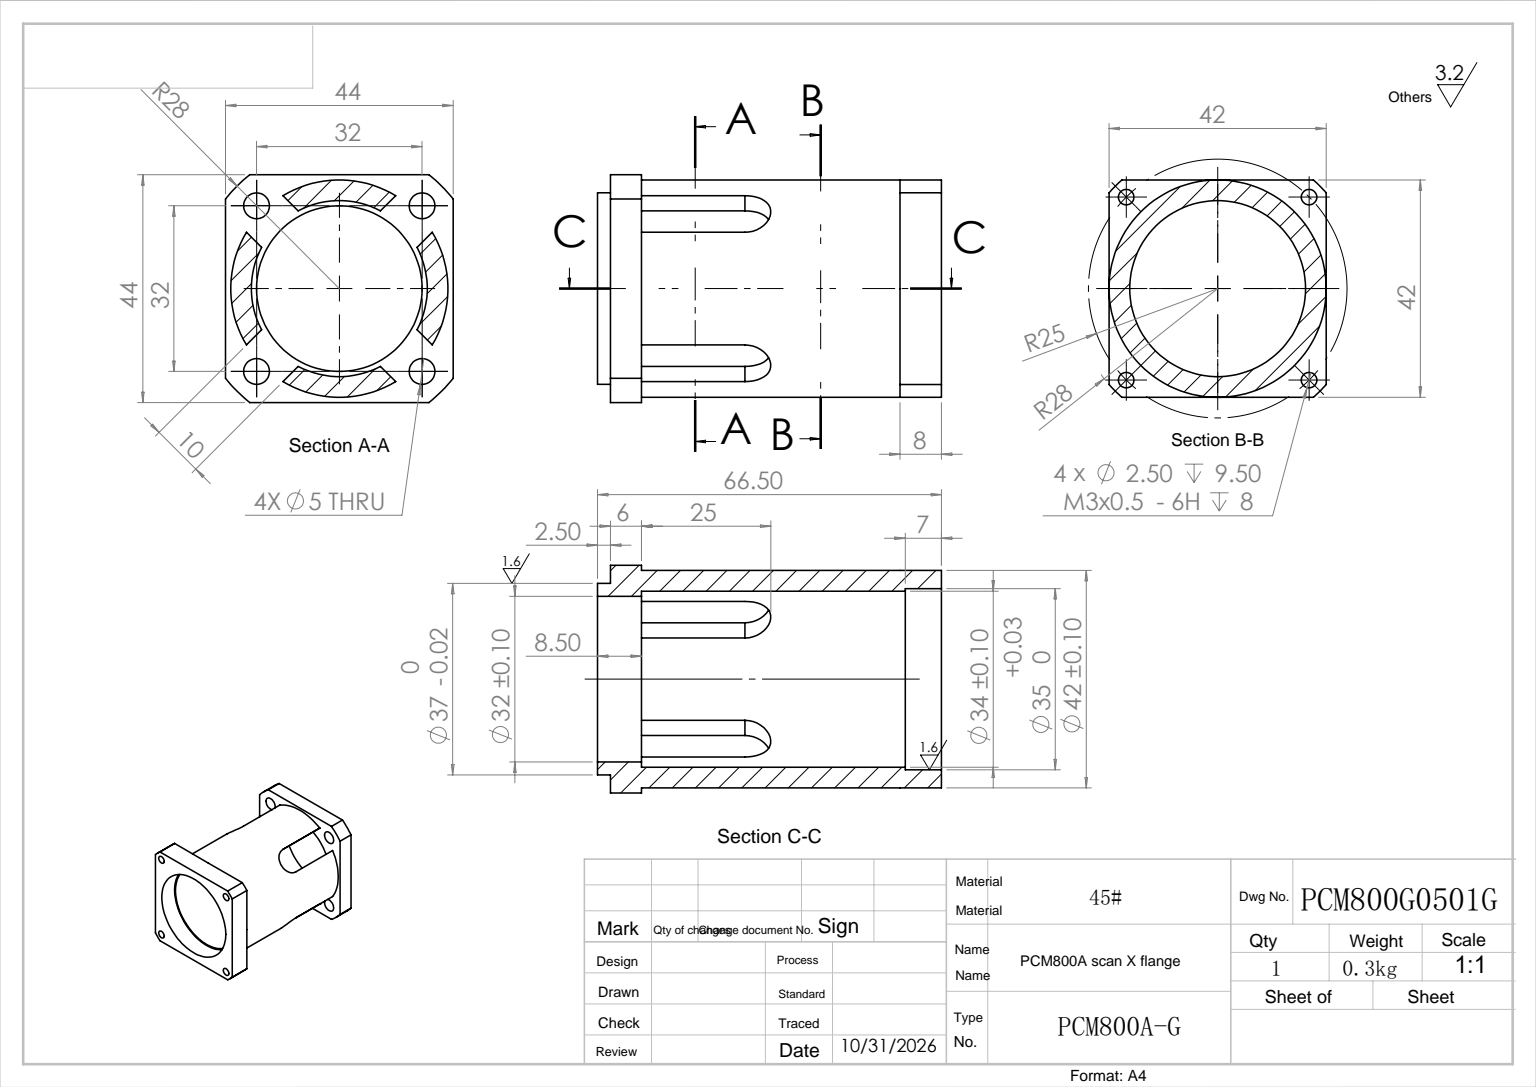
SolidWorks part; units mm, degrees
ref_plane "前视" through (0, 0, 0) normal (0, 0, 1) x (1, 0, 0)
ref_plane "上视" through (0, 0, 0) normal (0, 1, 0) x (1, 0, 0)
ref_plane "右视" through (0, 0, 0) normal (1, 0, 0) x (0, 0, -1)
sketch "草图1" plane through (0, 0, 0) normal (0, 0, 1) x (1, 0, 0)
  circle A0 centre (0, 0) radius 21
  circle A1 centre (0, 0) radius 17
  dimension "D1" = 42
  dimension "D2" = 34
extrude "拉伸1" add sketch "草图1" along normal blind 50
sketch "草图3" plane through (0, 0, 0) normal (0, 0, -1) x (-1, 0, 0)
  line L0 (0, 27.9971) -> (0, -28.1043) construction
  line L1 (-24.189, 0) -> (27.5144, 0) construction
  line L3 (-22, 22) -> (22, 22)
  line L4 (-22, 22) -> (-22, -22)
  line L5 (-22, -22) -> (22, -22)
  line L6 (22, 22) -> (22, -22)
  dimension "D1" = 22
  dimension "D2" = 22
  dimension "D3" = 44
  dimension "D4" = 44
extrude "拉伸2" add sketch "草图3" along normal blind 6
sketch "草图4" plane through (0, 0, -6) normal (0, 0, -1) x (-1, 0, 0)
  line L0 (-22, 0) -> (22, 0) construction
  line L1 (-22, 22) -> (-22, -22) construction
  line L2 (22, -22) -> (22, 22) construction
  line L3 (0, 22) -> (0, -22) construction
  line L4 (22, 22) -> (-22, 22) construction
  line L5 (-22, -22) -> (22, -22) construction
  line L6 (0, 0) -> (-22, 22) construction
  circle A0 centre (-16, 16) radius 2.5
  circle A1 centre (16, 16) radius 2.5
  circle A2 centre (16, -16) radius 2.5
  circle A3 centre (-16, -16) radius 2.5
  dimension "D1" = 5
  dimension "D2" = 16
extrude "切除-拉伸2" cut sketch "草图4" against normal up to surface (6 mm away) up to face at (0, 0, 0)
sketch "草图5" plane through (0, 0, 50) normal (0, 0, 1) x (1, 0, 0)
  line L1 (-21, 21) -> (21, 21)
  line L2 (-21, 21) -> (-21, -21)
  line L3 (-21, -21) -> (21, -21)
  line L4 (21, 21) -> (21, -21)
  circle A0 centre (0, 0) radius 21 construction
extrude "拉伸3" add sketch "草图5" along normal blind 8
sketch "草图6" plane through (0, 0, -6) normal (0, 0, -1) x (-1, 0, 0)
  circle A0 centre (0, 0) radius 18.5
  dimension "D1" = 37
extrude "拉伸4" add sketch "草图6" along normal blind 2.5
sketch "草图7" plane through (0, 0, 58) normal (0, 0, 1) x (1, 0, 0)
  circle A0 centre (0, 0) radius 17
  dimension "D1" = 34
extrude "切除-拉伸3" cut sketch "草图7" against normal up to next
sketch "草图8" plane through (0, 0, 58) normal (0, 0, 1) x (1, 0, 0)
  circle A0 centre (0, 0) radius 17.5
  dimension "D1" = 35
extrude "切除-拉伸4" cut sketch "草图8" against normal blind 7
sketch "草图9" plane through (0, 0, 58) normal (0, 0, 1) x (1, 0, 0)
  line L0 (-21, 0) -> (21, 0) construction
  line L1 (21, -21) -> (21, 21) construction
  line L2 (0, -21) -> (0, 21) construction
  line L3 (-21, -21) -> (21, -21) construction
  line L4 (21, 21) -> (-21, 21) construction
  line L5 (0, 0) -> (-21, 21) construction
  line L6 (21, 21) -> (-21, -21) construction
  line L7 (0, 0) -> (21, -21) construction
hole_wizard "M3x0.5 螺纹孔1" positions "3D草图3" profile "草图10" tap size "M3x0.5" standard "Ansi Metric"
sketch3d "3D草图3"
  line L0 (0, 0, 58) -> (-21, 21, 58) construction
  line L1 (21, 21, 58) -> (-21, -21, 58) construction
  line L3 (0, 0, 58) -> (21, -21, 58) construction
  point P0 (-17.6777, 17.6777, 58)
  point P4 (17.6777, 17.6777, 58)
  point P9 (-17.6777, -17.6777, 58)
  point P10 (17.6777, -17.6777, 58)
  dimension "D1" = 25
  dimension "D2" = 25
  dimension "D3" = 25
sketch "草图10" plane through (-17.6777, 17.6777, 58) normal (1, 0, 0) x (0, -1, 0)
  line L0 (0, 0) -> (0, 10.2511)
  line L1 (0, 10.2511) -> (1.25, 9.5)
  line L2 (1.25, 9.5) -> (1.25, 8)
  line L3 (1.25, 8) -> (1.5, 8)
  line L4 (1.5, 8) -> (1.5, 0)
  line L5 (1.5, 0) -> (0, 0)
  line L10 (0, 10.2511) -> (-1.25, 9.5) construction
  line L11 (0, -6.35) -> (0, 107.95) construction
  dimension "蹟恇謂郰芛眻噤" = 2.5
  dimension "蹟恇謂郰芛旮僅" = 9.5
  dimension "蹟恇翋眻噤" = 3
  dimension "蹟恇旮僅" = 8
  dimension "絳芛褒僅" = 118
ref_plane "基准面2" through (21, 21, 58) normal (-0.7071, -0.7071, 0) x (0.7071, -0.7071, 0)
sketch "草图11" plane through (21, 21, 58) normal (-0.7071, -0.7071, 0) x (0.7071, -0.7071, 0)
  line L0 (0, 0) -> (0, -65.2036) construction
  line L1 (-5, -38) -> (-5, -58)
  line L2 (-5, -58) -> (5, -58)
  line L5 (5, -38) -> (5, -58)
  line L6 (31.1127, -58) -> (0, -58) construction
  arc A0 (5, -38) -> (-5, -38) centre (0, -38) ccw
  dimension "D1" = 10
  dimension "D2" = 20
  dimension "D3" = 10
extrude "切除-拉伸6" cut sketch "草图11" along normal through all
ref_plane "基准面3" through (21, -21, 58) normal (0.7071, -0.7071, 0) x (0.7071, 0.7071, 0)
sketch "草图12" plane through (21, -21, 58) normal (0.7071, -0.7071, 0) x (0.7071, 0.7071, 0)
  line L0 (0, 0) -> (0, -44.1526) construction
  line L1 (0, -58) -> (-31.1127, -58) construction
  line L2 (-5, -38) -> (-5, -58)
  line L3 (5, -38) -> (5, -58)
  line L4 (-5, -58) -> (5, -58)
  arc A0 (5, -38) -> (-5, -38) centre (0, -38) ccw
  dimension "D2" = 20
  dimension "D1" = 10
extrude "切除-拉伸7" cut sketch "草图12" against normal through all
sketch "草图13" plane through (0, 0, -8.5) normal (0, 0, -1) x (-1, 0, 0)
  circle A0 centre (0, 0) radius 16
  dimension "D1" = 32
extrude "切除-拉伸8" cut sketch "草图13" against normal up to next
sketch "草图14" plane through (0, 0, 58) normal (0, 0, 1) x (1, 0, 0)
  circle A0 centre (0, 0) radius 28
  dimension "D1" = 56
extrude "切除-拉伸9" cut sketch "草图14" against normal through all flip side to cut
